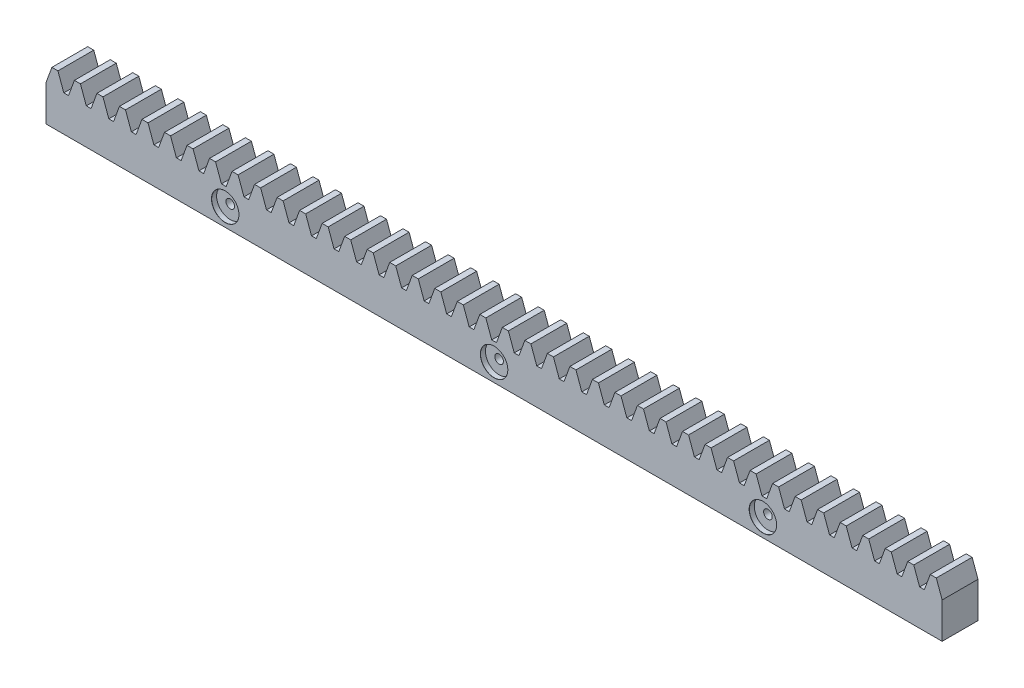
SolidWorks part; units mm, degrees
ref_plane "Front Plane" through (0, 0, 0) normal (0, 0, 1) x (1, 0, 0)
ref_plane "Top Plane" through (0, 0, 0) normal (0, 1, 0) x (1, 0, 0)
ref_plane "Right Plane" through (0, 0, 0) normal (1, 0, 0) x (0, 0, -1)
sketch "Sketch1" plane through (0, 0, 0) normal (0, 0, 1) x (1, 0, 0)
  line L1 (0, 0) -> (250, 0)
  line L2 (0, 0) -> (0, -10)
  line L3 (0, -10) -> (250, -10)
  line L4 (250, 0) -> (250, -10)
extrude "Extrude1" add sketch "Sketch1" along normal blind 10
sketch "Sketch2" plane through (0, 0, 10) normal (0, 0, 1) x (1, 0, 0)
  line L0 (0, 0) -> (1.6379, 4.5)
  line L1 (1.6379, 4.5) -> (3.3236, 4.5)
  line L2 (3.3236, 4.5) -> (4.9614, 0)
  line L3 (250, 0) -> (0, 0) construction
  line L4 (0, 0) -> (4.9614, 0)
  line L5 (0.9099, 2.5) -> (4.0515, 2.5) construction
extrude "Extrude2" add sketch "Sketch2" against normal up to surface (10 mm away) up to face at (125, -5, 0)
pattern_linear "LPattern1" count 40 spacing 6.2832 along (1, 0, 0) of "Extrude2"
sketch "Sketch3" plane through (0, 0, 10) normal (0, 0, 1) x (1, 0, 0)
  line L0 (48.0338, 2.5) -> (51.1754, 2.5) construction
  line L3 (53.5891, 4.5) -> (51.9033, 4.5) construction
  line L4 (199.2897, 2.5) -> (201.5352, 2.5) construction
  line L5 (204.3855, 4.5) -> (202.6998, 4.5) construction
  dimension "D1" = 2
  dimension "D2" = 2
sketch "Sketch5" plane through (0, 0, 10) normal (0, 0, 1) x (1, 0, 0)
  line L0 (0, -10) -> (250, -10) construction
  line L1 (0, 0) -> (0, -10) construction
  line L2 (250, -10) -> (250, 0) construction
  line L3 (50, -5) -> (125, -5)
  line L4 (200, -5) -> (250, -5)
  dimension "D1" = 5
  dimension "D3" = 50
  dimension "D5" = 75
  dimension "D2" = 50
  dimension "D4" = 5
  dimension "D6" = 150
  dimension "D7" = 5
hole_wizard "CBORE for M2 Hex Cap Screw1" positions "Sketch12" profile "Sketch13" counterbore size "M2" standard "ISO"
sketch "Sketch12" plane through (0, 0, 10) normal (0, 0, 1) x (1, 0, 0)
  point P0 (50, -5)
  point P3 (125, -5)
  point P6 (200, -5)
sketch "Sketch13" plane through (50, -5, 10) normal (1, 0, 0) x (0, -1, 0)
  line L0 (0, 0) -> (0, 15.721)
  line L1 (0, 15.721) -> (1.2, 15)
  line L2 (1.2, 15) -> (1.2, 1.4)
  line L3 (1.2, 1.4) -> (3.8095, 1.4)
  line L5 (3.8095, 1.4) -> (3.8095, 0.025)
  line L6 (3.8095, 0.025) -> (3.8345, 0)
  line L7 (3.8345, 0) -> (0, 0)
  line L8 (-3.8095, 0.025) -> (-3.8345, 0) construction
  line L10 (0, 15.721) -> (-1.2, 15) construction
  line L11 (0, -6.35) -> (0, 107.95) construction
  dimension "孔直径" = 2.4
  dimension "孔深度" = 15
  dimension "锥形沉头孔直径" = 7.619
  dimension "锥形沉头孔深度" = 1.4
  dimension "近端锥形沉头孔直径" = 7.669
  dimension "近端锥形沉头孔角度" = 90
  dimension "导头角度" = 118
equation "\"d\"=\"S@Sketch2\" * 2"
equation "\"z\"= int(  \"L@Sketch1\" / (  \"S@Sketch2\" * 2 ) + 0.5 )"
